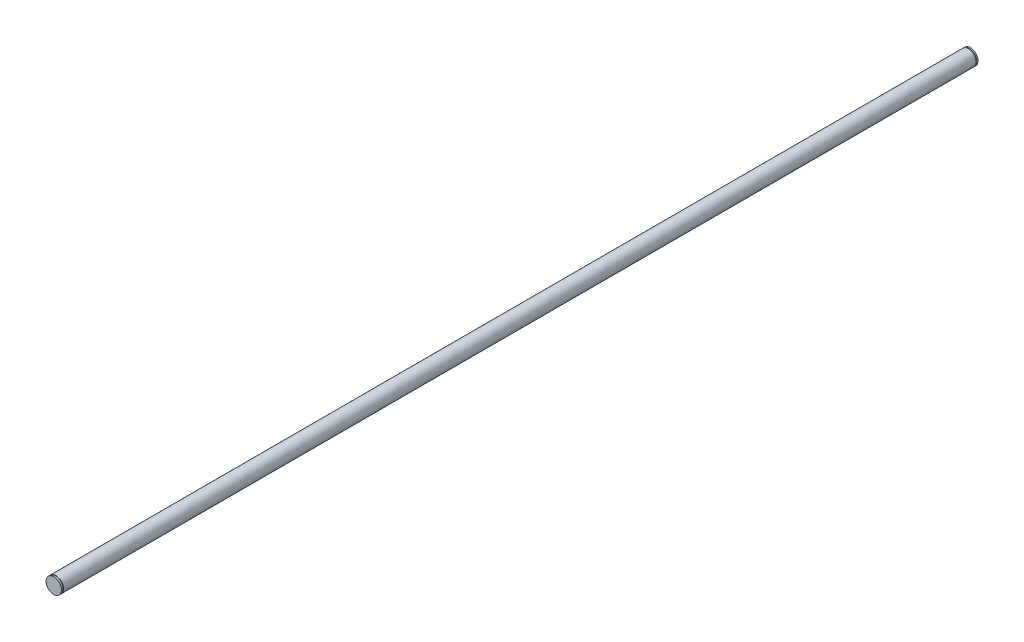
SolidWorks part; units mm, degrees
ref_plane "前视基准面" through (0, 0, 0) normal (0, 0, 1) x (1, 0, 0)
ref_plane "上视基准面" through (0, 0, 0) normal (0, 1, 0) x (1, 0, 0)
ref_plane "右视基准面" through (0, 0, 0) normal (1, 0, 0) x (0, 0, -1)
sketch "草图1" plane through (0, 0, 0) normal (0, 0, 1) x (1, 0, 0)
  circle A0 centre (0, 0) radius 12.5
  dimension "D1" = 25
extrude "凸台-拉伸1" add sketch "草图1" along normal blind 1470
sketch "草图9" plane through (0, 0, 0) normal (0, 0, -1) x (-1, 0, 0)
  circle A1 centre (0, 0) radius 12.5
  circle A2 centre (0, 0) radius 12.5
  dimension "D1" = 0
extrude "凸台-拉伸5" add sketch "草图9" along normal blind 50
ref_plane "基准面1" through (0, 0, 710) normal (0, 0, 1) x (1, 0, 0)
sketch "草图2" plane through (0, 0, 0) normal (0, 1, 0) x (1, 0, 0)
  line L0 (12.5, -1470) -> (12.5, 50) construction
  line L1 (12.5, -1450) -> (11.95, -1450)
  line L2 (12.5, -1450) -> (12.5, -1451.3)
  line L3 (12.5, -1451.3) -> (11.95, -1451.3)
  line L4 (11.95, -1450) -> (11.95, -1451.3)
  line L5 (-11.95, -1450) -> (-11.95, -1451.3)
  line L6 (0, -1476.0334) -> (0, -1496.066) construction
  line L7 (-12.5, -1451.3) -> (-11.95, -1451.3)
  line L8 (12.5, -710) -> (150.7089, -710) construction
  line L9 (-12.5, -1450) -> (-12.5, -1451.3)
  line L10 (-12.5, -1450) -> (-11.95, -1450)
  line L11 (0, 56.0334) -> (0, 76.066) construction
  line L12 (-12.5, 30) -> (-11.95, 30)
  line L13 (-12.5, 30) -> (-12.5, 31.3)
  line L14 (-12.5, 31.3) -> (-11.95, 31.3)
  line L15 (-11.95, 30) -> (-11.95, 31.3)
  line L16 (11.95, 30) -> (11.95, 31.3)
  line L17 (12.5, 31.3) -> (11.95, 31.3)
  line L18 (12.5, 30) -> (12.5, 31.3)
  line L19 (12.5, 30) -> (11.95, 30)
  dimension "D1" = 1.3
  dimension "D2" = 0.55
  dimension "D3" = 740
  dimension "D4" = 12.5
revolve "切除-旋转1" cut sketch "草图2" angle 360 about L6
sketch "草图11" plane through (0, 0, 1470) normal (0, 0, 1) x (1, 0, 0)
  circle A1 centre (0, 0) radius 12.5
  circle A2 centre (0, 0) radius 12.5
  dimension "D1" = 0
extrude "切除-拉伸2" cut sketch "草图11" against normal blind 16.5
sketch "草图12" plane through (0, 0, -50) normal (0, 0, -1) x (-1, 0, 0)
  circle A1 centre (0, 0) radius 12.5
  circle A2 centre (0, 0) radius 12.5
  dimension "D1" = 0
extrude "切除-拉伸3" cut sketch "草图12" against normal blind 16.5
